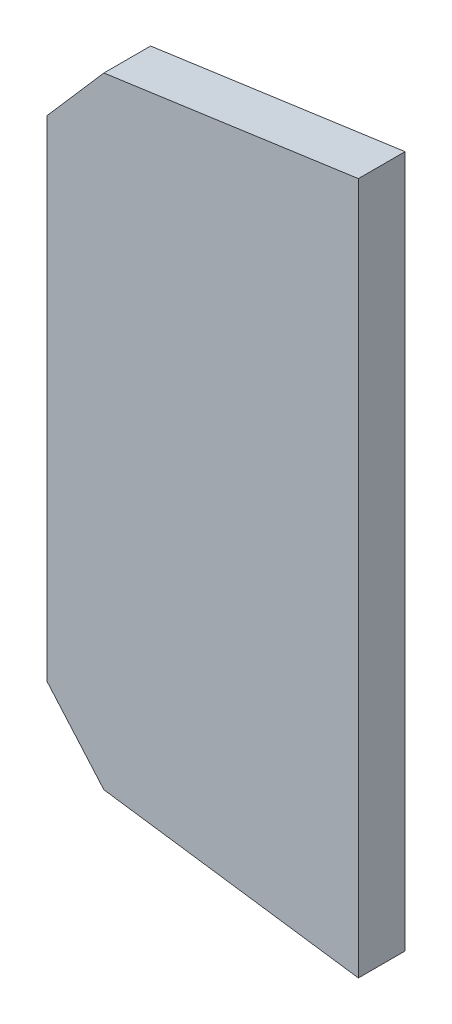
SolidWorks part; units mm, degrees
material "1023 Carbon Steel Plate (SS)"
ref_plane "Front Plane" through (0, 0, 0) normal (0, 0, 1) x (1, 0, 0)
ref_plane "Top Plane" through (0, 0, 0) normal (0, 1, 0) x (1, 0, 0)
ref_plane "Right Plane" through (0, 0, 0) normal (1, 0, 0) x (0, 0, -1)
sketch "Sketch1" plane through (0, 0, 0) normal (0, 0, 1) x (1, 0, 0)
  line L4 (-4, -94.4514) -> (-36.683, -89.8581)
  line L5 (-44, -81.4408) -> (-44, -18.5592)
  line L6 (-36.683, -10.1419) -> (-4, -5.5486)
  line L9 (-4, -5.5486) -> (-4, -94.4514)
  line L10 (-36.683, -10.1419) -> (-44, -18.5592)
  line L11 (-44, -81.4408) -> (-36.683, -89.8581)
  dimension "D10" = 40
extrude "Boss-Extrude1" add sketch "Sketch1" along normal blind 6 contours L4 L11 L5 L10 L6 L9
